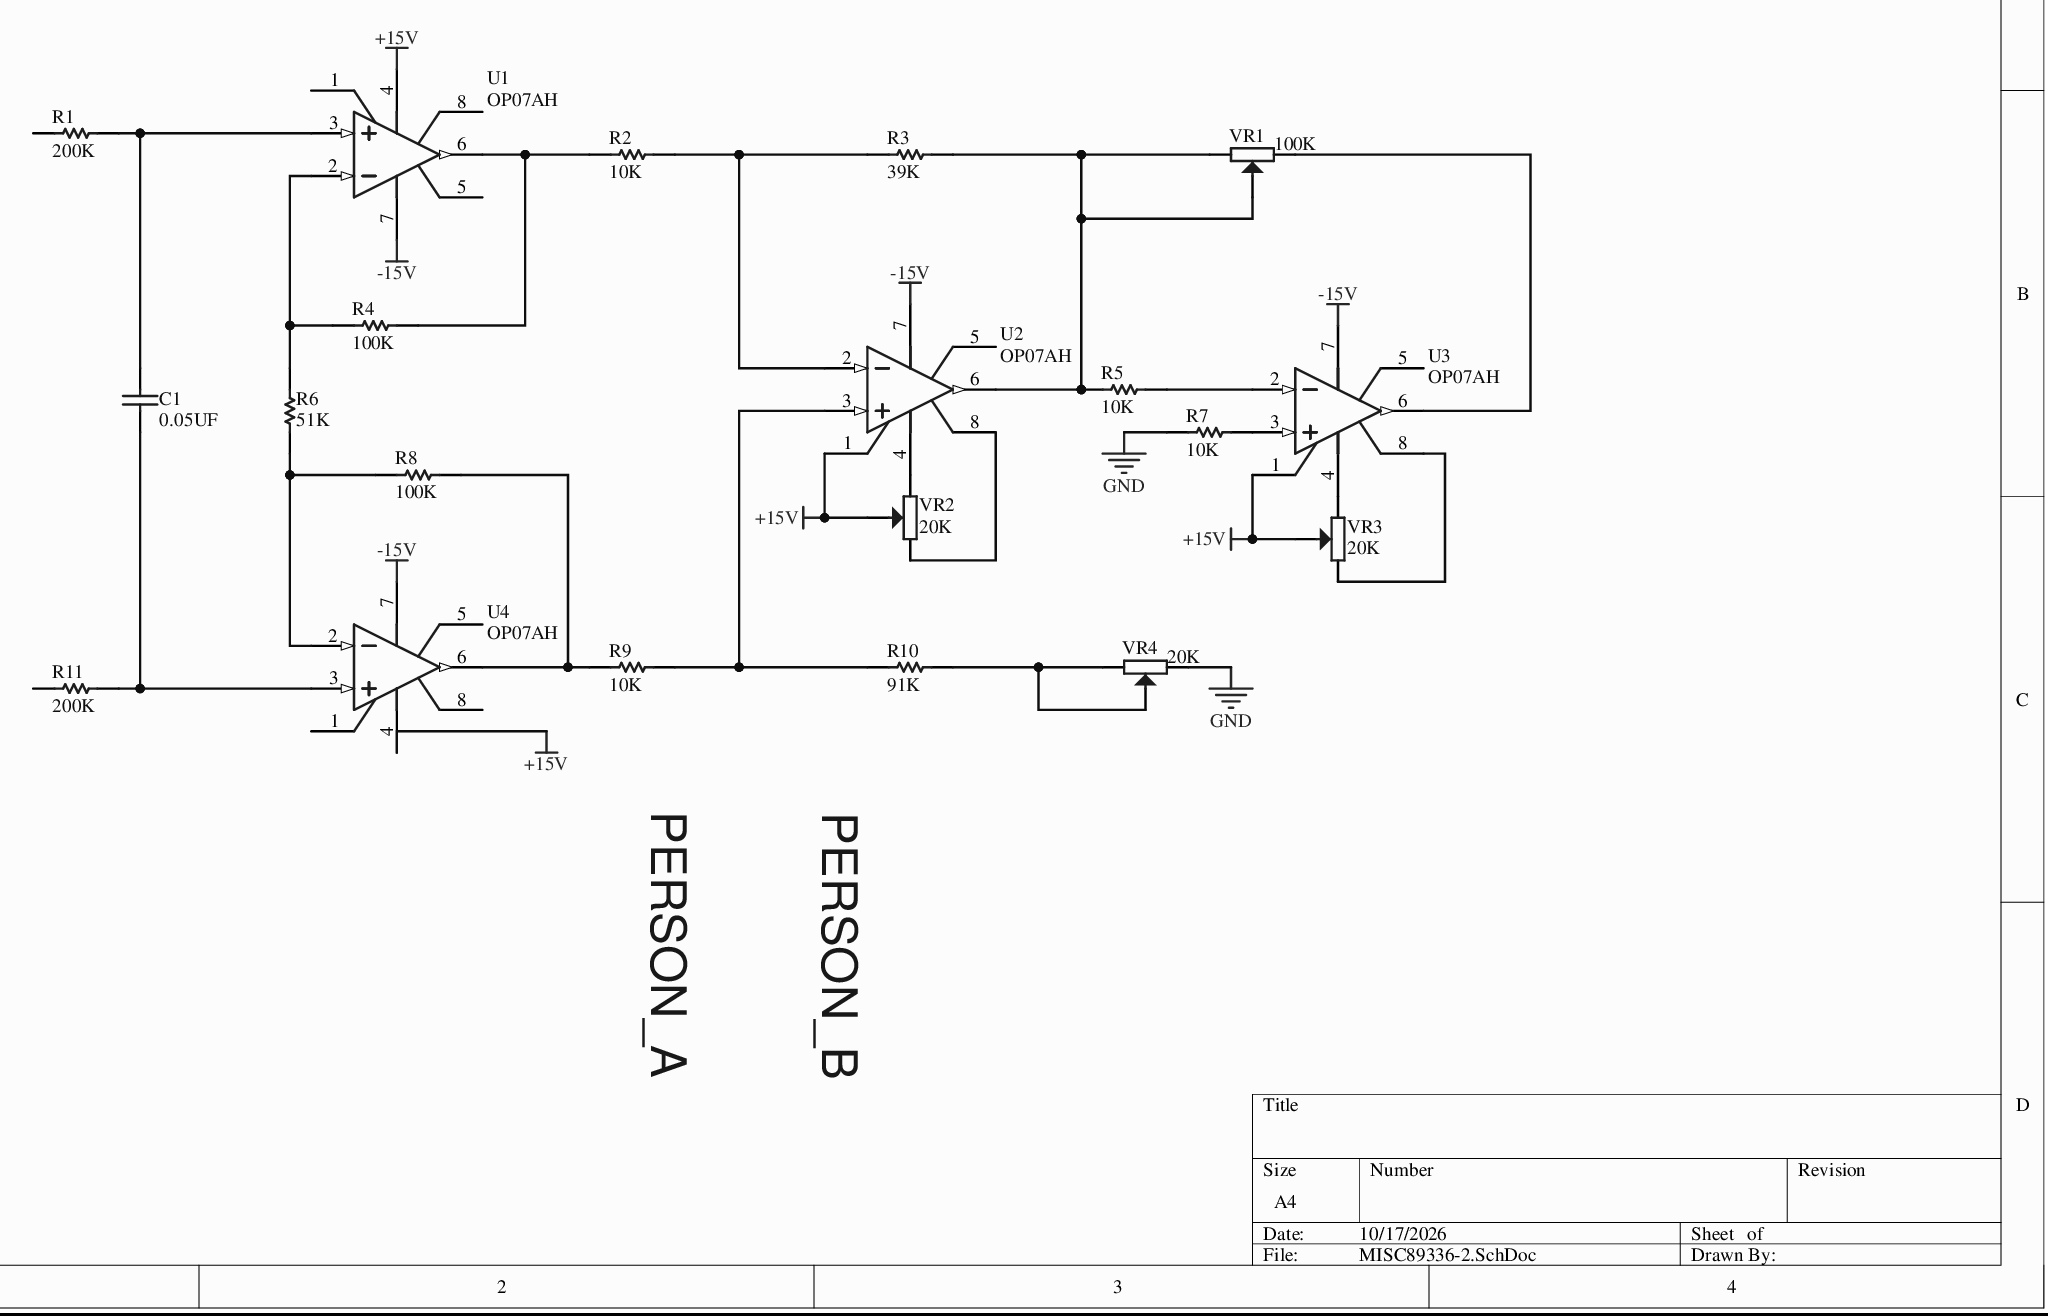
[diagram p0: MISC89336-2.SchDoc]
# Altium project MISC89336-3.PrjPcb
1 sheet, 20 parts. Net scope: global (net labels, ports and power ports of the same name join across sheets).
Board file: MISC89336.PcbDoc

## Sheet MISC89336-2.SchDoc
size A4

### Parts
C1  0.05UF  [C2512]
R1  200K  [AXIAL0.4]
R2  10K  [AXIAL0.4]
R3  39K  [AXIAL0.4]
R4  100K  [AXIAL0.4]
R5  10K  [AXIAL0.4]
R6  51K  [AXIAL0.4]
R7  10K  [AXIAL0.4]
R8  100K  [AXIAL0.4]
R9  10K  [AXIAL0.4]
R10  91K  [AXIAL0.4]
R11  200K  [AXIAL0.4]
U1  OP07AH  [DIP8]
U2  OP07AH  [DIP8]
U3  OP07AH  [DIP8]
U4  OP07AH  [DIP8]
VR1  100K  [3296W]
VR2  20K  [3296W]
VR3  20K  [3296W]
VR4  20K  [3296W]

### Nets
+15V: U1.4(V-) U2.1(OS_NULL) U3.1(OS_NULL) U4.4(V-) VR2.2 VR3.2
-15V: U1.7(V+) U2.7(V+) U3.7(V+) U4.7(V+)
GND: R7.1 VR4.1
NetC1_1: C1.1 R11.2 U4.3(IN+)
NetC1_2: C1.2 R1.2 U1.3(IN+)
NetR2_1: R2.1 R4.2 U1.6(OUT)
NetR2_2: R2.2 R3.1 U2.2(IN-)
NetR3_2: R3.2 R5.1 U2.6(OUT) VR1.2
NetR4_1: R4.1 R6.2 U1.2(IN-)
NetR5_2: R5.2 U3.2(IN-)
NetR6_1: R6.1 R8.1 U4.2(IN-)
NetR7_2: R7.2 U3.3(IN+)
NetR8_2: R8.2 R9.1 U4.6(OUT)
NetR9_2: R9.2 R10.1 U2.3(IN+)
NetR10_2: R10.2 VR4.2
NetU2_4: U2.4(V-) VR2.2
NetU2_8: U2.8(OS_NULL) VR2.1
NetU3_4: U3.4(V-) VR3.2
NetU3_6: U3.6(OUT) VR1.1
NetU3_8: U3.8(OS_NULL) VR3.1

Not connected (* = marked no-connect by the designer): R1 1; R11 1; U1 1(OS_NULL) 5(NC) 8(OS_NULL); U2 5(NC); U3 5(NC); U4 1(OS_NULL) 5(NC) 8(OS_NULL)

### Notes on the sheet
- PERSON_A
- PERSON_B

### Library data of the parts
C1 = Cap Semi: Capacitor (Semiconductor SIM Model); Value: 100pF; Published: 8-Jun-2000; LatestRevisionDate: 29-May-2009; LatestRevisionNote: IPC-7351 Footprint Added.; PackageReference: C1206; PackageDescription: Chip Capacitor; Publisher: Altium Limited
R1-R11 = RES
U1-U4 = ADOP07AH: Ultra-Low Offset Voltage Operational Amplifier; Package Information: Latest Revision: 1990; Note: Pin 5 is not connected.; Published: 8-Jun-2000; Revision: 17-Jul-2002: Re-released for DXP Platform.; Datasheet: Amplifier Reference Manual (1992); Package Reference: H-08A; Publisher: Altium Limited
VR1-VR4 = RESVR